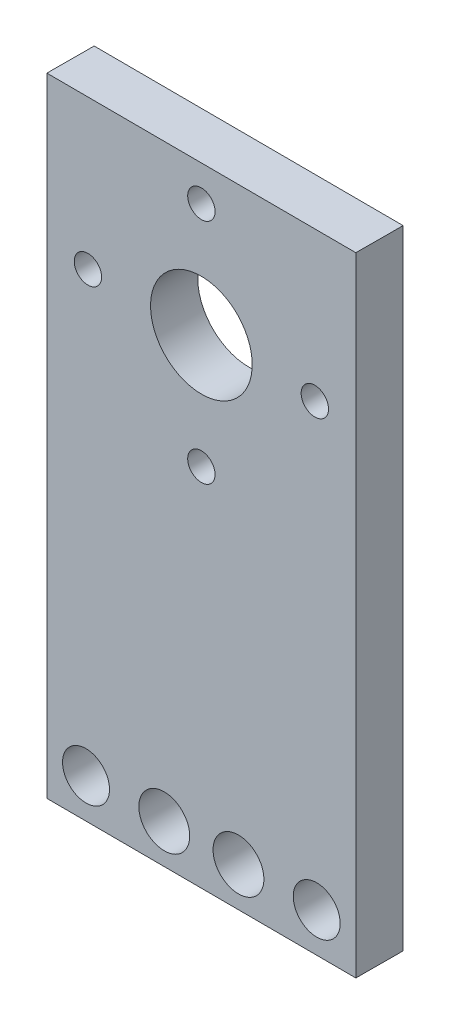
SolidWorks part; units mm, degrees
ref_plane "前视基准面" through (0, 0, 0) normal (0, 0, 1) x (1, 0, 0)
ref_plane "上视基准面" through (0, 0, 0) normal (0, 1, 0) x (1, 0, 0)
ref_plane "右视基准面" through (0, 0, 0) normal (1, 0, 0) x (0, 0, -1)
sketch "草图2" plane through (0.0318, 0, -9.2899) normal (-0.0034, 0, 1) x (1, 0, 0.0034)
  line L0 (-185.5205, -9.8708) -> (-185.5205, 70.1292) construction
  line L2 (-205.5205, -9.8708) -> (-166.0371, -9.8708)
  line L3 (-166.0371, -9.8708) -> (-166.0371, 70.1292)
  line L4 (-205.5205, -9.8708) -> (-205.5205, 70.1292)
  line L5 (-205.5205, 70.1292) -> (-166.0371, 70.1292)
  line L6 (-166.0371, -9.8708) -> (-166.0371, 38.2917) construction
  line L7 (-205.5205, -9.8708) -> (-205.5205, 38.2917) construction
  line L8 (-185.5205, -9.8708) -> (-185.5205, 38.2917) construction
  dimension "D1" = 80
extrude "凸台-拉伸1" add sketch "草图2" along normal blind 6
ref_plane "基准面4" through (-185.7777, 0, -0.6368) normal (1, 0, 0.0034) x (0.0034, 0, -1)
sketch "草图3" plane through (0.0113, 0, -3.2899) normal (-0.0034, 0, 1) x (1, 0, 0.0034)
  line L0 (-205.5205, -4.8708) -> (-166.0371, -4.8708) construction
  line L1 (-205.5205, 70.1292) -> (-205.5205, -9.8708) construction
  line L2 (-166.0371, -9.8708) -> (-166.0371, 70.1292) construction
  line L3 (-200.5205, 1.458) -> (-200.5205, -4.8708) construction
  line L4 (-171.0371, 1.458) -> (-171.0371, -4.8708) construction
  line L5 (-205.5205, -9.8708) -> (-166.0371, -9.8708) construction
  circle A0 centre (-200.5205, -4.8708) radius 3
  circle A1 centre (-171.0371, -4.8708) radius 3
  dimension "D4" = 6
  dimension "D5" = 6
  dimension "D1" = 5
  dimension "D2" = 5
  dimension "D3" = 5
extrude "切除-拉伸1" cut sketch "草图3" against normal blind 10
hole_wizard "Ø1.0 (1) 直径孔1" positions "草图4" profile "草图5" hole size "Ø1.0" standard "GB" end condition through all
sketch "草图4" plane through (0.0113, 0, -3.2899) normal (-0.0034, 0, 1) x (1, 0, 0.0034)
  line L0 (-205.5205, -9.8708) -> (-166.0371, -9.8708) construction
  circle A0 centre (-200.5205, -4.8708) radius 3 construction
  circle A1 centre (-171.0371, -4.8708) radius 3 construction
  point P0 (-190.5205, -4.8708)
  point P2 (-181.0371, -4.8708)
  dimension "D1" = 5
  dimension "D2" = 5
  dimension "D3" = 10
  dimension "D4" = 10
sketch "草图5" plane through (-190.5081, -4.8708, -3.943) normal (0, 1, 0) x (1, 0, 0.0034)
  line L0 (0, 0) -> (0, 6.1353)
  line L1 (0, 6.1353) -> (3.25, 6.1353)
  line L2 (3.25, 6.1353) -> (3.25, 0)
  line L5 (3.25, 0) -> (0, 0)
  line L11 (0, -6.35) -> (0, 107.95) construction
  dimension "通孔孔直径" = 6.5
  dimension "通孔孔深度" = 6.1353
sketch "草图6" plane through (0.0318, 0, -9.2899) normal (0.0034, 0, -1) x (-1, 0, -0.0034)
  circle A0 centre (185.7776, 51.1292) radius 6.5
extrude "切除-拉伸2" cut sketch "草图6" against normal through all
hole_wizard "Ø1.0 (1) 直径孔2" positions "草图7" profile "草图8" hole size "Ø1.0" standard "GB" end condition through all
sketch "草图7" plane through (0.0113, 0, -3.2899) normal (-0.0034, 0, 1) x (1, 0, 0.0034)
  point P0 (-185.7776, 65.6292)
  point P2 (-171.2776, 51.1292)
  point P4 (-185.7776, 36.6292)
  point P6 (-200.2776, 51.1292)
sketch "草图8" plane through (-185.7652, 65.6292, -3.9267) normal (0, 1, 0) x (1, 0, 0.0034)
  line L0 (0, 0) -> (0, 6.1353)
  line L1 (0, 6.1353) -> (1.75, 6.1353)
  line L2 (1.75, 6.1353) -> (1.75, 0)
  line L5 (1.75, 0) -> (0, 0)
  line L11 (0, -6.35) -> (0, 107.95) construction
  dimension "通孔孔直径" = 3.5
  dimension "通孔孔深度" = 6.1353
ref_plane "基准面5" through (-185.7777, 0, -0.6368) normal (1, 0, 0.0034) x (0.0034, 0, -1)
ref_plane "基准面6" through (-185.7777, 0, -0.6368) normal (-1, 0, -0.0034) x (-0.0034, 0, 1)
